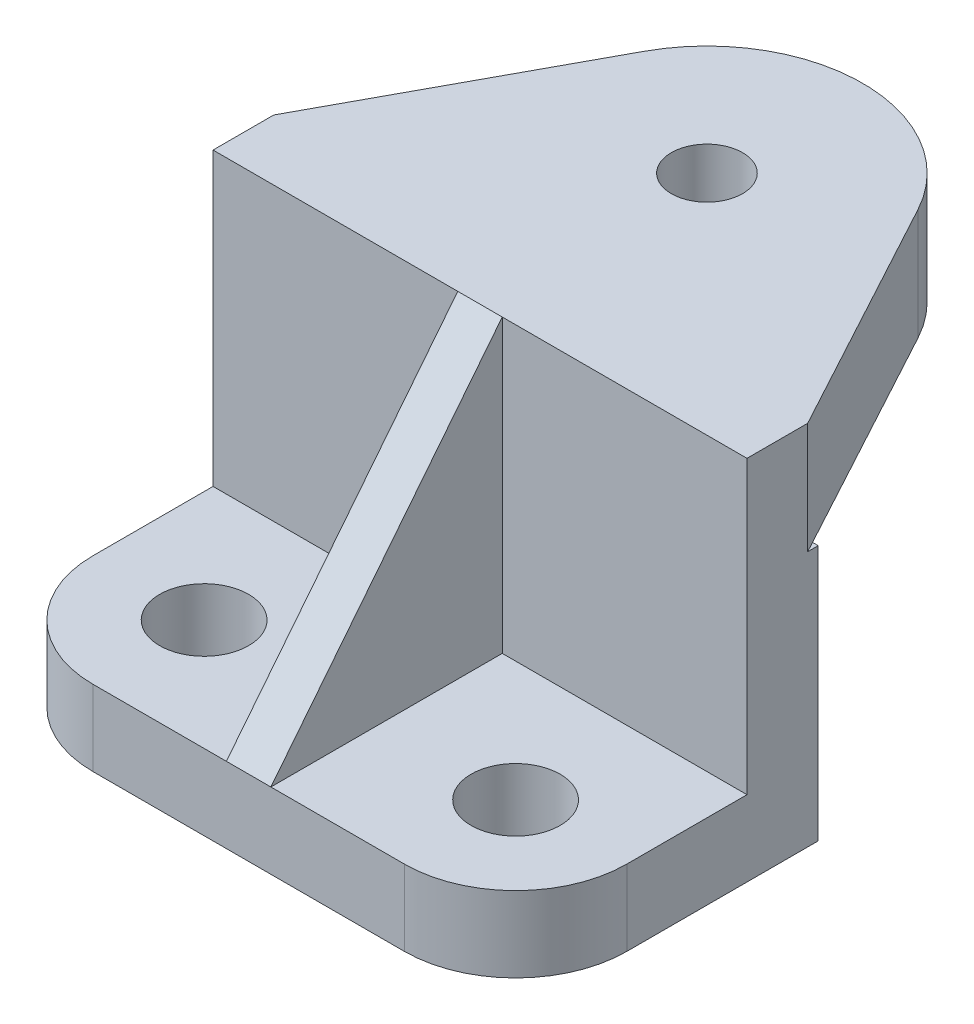
from build123d import *

# Parameters (mm, degrees)
BOSS_EXTRUDE1_DEPTH = 120
CUT_EXTRUDE1_DEPTH  = 55
CUT_EXTRUDE2_DEPTH  = 55
SKETCH5_R           = 10
CUT_EXTRUDE3_DEPTH  = 55
SKETCH6_W           = 70
SKETCH6_H           = 25
BOSS_EXTRUDE2_DEPTH = 120
SKETCH7_R           = 8
CUT_EXTRUDE4_DEPTH  = 25


with BuildPart() as part:
    # Sketch1 → Boss-Extrude1 (new body)
    with BuildSketch(Plane(origin=(0, 0, 0), x_dir=(0, 0, -1), z_dir=(1, 0, 0))):
        Polygon((52, 82.471222814), (52, 17), (0, 17), align=None)
        Polygon((52, 17), (0, 17), (0, 0), (68, 0), (68, 82.471222814), (52, 82.471222814), align=None)
    extrude(amount=-BOSS_EXTRUDE1_DEPTH)

    # Sketch2 → Cut-Extrude1 (cut)
    with BuildSketch(Plane(origin=(0, 0, 0), x_dir=(0, 0, -1), z_dir=(1, 0, 0))):
        Polygon((52, 82.471222814), (0, 17), (52, 17), align=None)
    extrude(amount=-CUT_EXTRUDE1_DEPTH, mode=Mode.SUBTRACT)

    # Sketch3 → Cut-Extrude2 (cut)
    with BuildSketch(Plane.ZY.offset(120)):
        Polygon((-52, 82.471222814), (0, 17), (-52, 17), align=None)
    extrude(amount=-CUT_EXTRUDE2_DEPTH, mode=Mode.SUBTRACT)

    # Sketch5 → Cut-Extrude3 (cut)
    with BuildSketch(Plane.XZ):
        with BuildLine():
            Line((-95, 0), (-120, 0))
            Line((-120, 0), (-120, -25))
            ThreePointArc((-120, -25), (-112.67766953, -7.32233047), (-95, 0))
        make_face()
        with Locations(Location((-95, -25, 0), (0, 0, 270))):
            Circle(SKETCH5_R)
        with BuildLine():
            Line((0, 0), (-25, 0))
            ThreePointArc((-25, 0), (-7.32233047, -7.32233047), (0, -25))
            Line((0, -25), (0, 0))
        make_face()
        with Locations(Location((-25, -25, 0), (0, 0, 270))):
            Circle(SKETCH5_R)
    extrude(amount=-CUT_EXTRUDE3_DEPTH, mode=Mode.SUBTRACT)

    # Sketch6 → Boss-Extrude2 (add)
    with BuildSketch(Plane(origin=(0, 0, 0), x_dir=(0, 0, -1), z_dir=(1, 0, 0))):
        with Locations((103, 69.971222814)):
            Rectangle(SKETCH6_W, SKETCH6_H)
    extrude(amount=-BOSS_EXTRUDE2_DEPTH)

    # Sketch7 → Cut-Extrude4 (cut)
    with BuildSketch(Plane(origin=(0, 82.471222814, 0), x_dir=(1, 0, 0), z_dir=(0, 1, 0))):
        with Locations(Location((-60, 103, 0), (0, 0, 270))):
            Circle(SKETCH7_R)
        with BuildLine():
            Line((0, 138), (-60, 138))
            ThreePointArc((-60, 138), (-42.081937118, 133.065645221), (-29.216107334, 119.653887004))
            Line((-29.216107334, 119.653887004), (0, 65.649346677))
            Line((0, 65.649346677), (0, 138))
        make_face()
        with BuildLine():
            Line((-120, 138), (-120, 65.649346677))
            Line((-120, 65.649346677), (-90.783892666, 119.653887004))
            ThreePointArc((-90.783892666, 119.653887004), (-77.918062882, 133.065645221), (-60, 138))
            Line((-60, 138), (-120, 138))
        make_face()
    extrude(amount=-CUT_EXTRUDE4_DEPTH, mode=Mode.SUBTRACT)


solid = part.part
